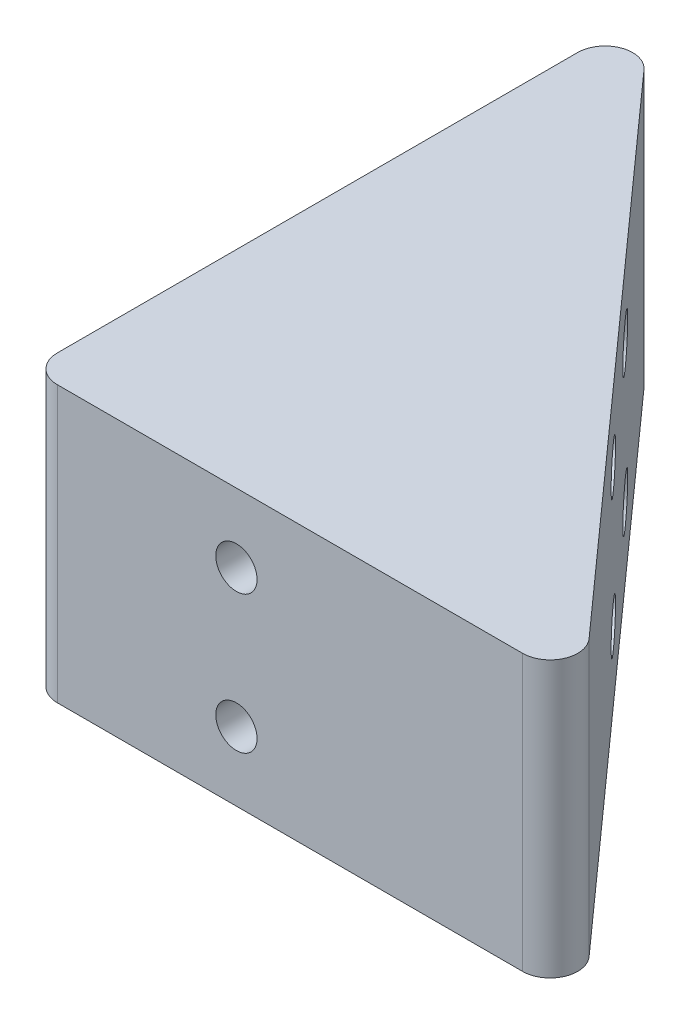
SolidWorks part; units mm, degrees
material "ABS"
ref_plane "前视基准面" through (0, 0, 0) normal (0, 0, 1) x (1, 0, 0)
ref_plane "上视基准面" through (0, 0, 0) normal (0, 1, 0) x (1, 0, 0)
ref_plane "右视基准面" through (0, 0, 0) normal (1, 0, 0) x (0, 0, -1)
other "Configuration Table"
sketch "草图1" plane through (0, 0, 0) normal (0, 1, 0) x (1, 0, 0)
  line L0 (0, 45) -> (0, 0)
  line L1 (0, 0) -> (40.2492, 0)
  line L2 (40.2492, 0) -> (0, 45)
  dimension "D1" = 30
  dimension "D2" = 45
extrude "凸台-拉伸1" add sketch "草图1" along normal blind 20
fillet "圆角1" radius 2 3 edges at (40.2492, 10, 0) (0, 10, -45) (0, 10, 0)
sketch "草图2" plane through (0, 0, 0) normal (-1, 0, 0) x (0, 0, 1)
  line L1 (-20, 15) -> (-20, 5) construction
  line L2 (-2, 0) -> (-2, 20) construction
  line L3 (0, 20) -> (0, 0) construction
  circle A0 centre (-20, 15) radius 1.5
  circle A1 centre (-20, 5) radius 1.5
  point P4 (-2, 10)
  point P7 (-20, 10)
  dimension "D1" = 10
  dimension "D3" = 3
  dimension "D2" = 20
extrude "切除-拉伸1" cut sketch "草图2" against normal through all
sketch "草图3" plane through (0, 0, 0) normal (0, 0, 1) x (1, 0, 0)
  line L0 (15, 15) -> (15, 5) construction
  line L1 (2, 20) -> (2, 0) construction
  line L2 (0, 0) -> (0, 20) construction
  circle A0 centre (15, 15) radius 1.5
  circle A1 centre (15, 5) radius 1.5
  point P6 (2, 10)
  point P7 (15, 10)
  dimension "D1" = 15
  dimension "D2" = 3
  dimension "D3" = 10
extrude "切除-拉伸2" cut sketch "草图3" against normal through all
